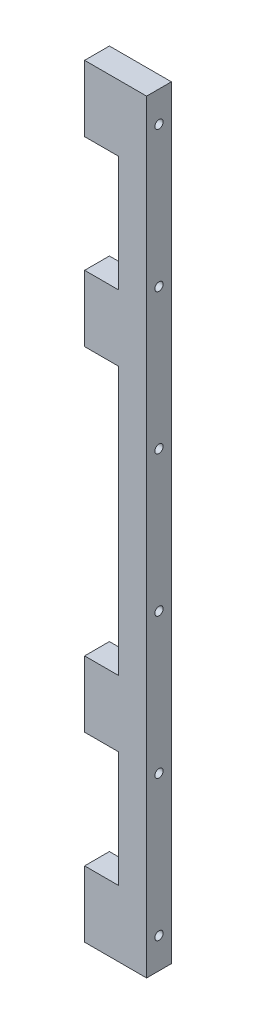
SolidWorks part; units mm, degrees
material "6061-T6"
ref_plane "前视基准面" through (0, 0, 0) normal (0, 0, 1) x (1, 0, 0)
ref_plane "上视基准面" through (0, 0, 0) normal (0, 1, 0) x (1, 0, 0)
ref_plane "右视基准面" through (0, 0, 0) normal (1, 0, 0) x (0, 0, -1)
sketch "草图1" plane through (0, 0, 0) normal (0, 0, 1) x (1, 0, 0)
  line L0 (23.5, 40) -> (23.5, 422) construction
  line L1 (0, 462) -> (40.5, 462)
  line L2 (0, 462) -> (0, 0)
  line L3 (0, 0) -> (40.5, 0)
  line L4 (40.5, 462) -> (40.5, 0)
  line L5 (0, 462) -> (23.5, 462)
  line L6 (0, 462) -> (0, 422)
  line L7 (0, 422) -> (23.5, 422)
  line L8 (23.5, 462) -> (23.5, 422) construction
  line L9 (0, 0) -> (23.5, 0)
  line L10 (0, 0) -> (0, 40)
  line L11 (0, 40) -> (23.5, 40)
  line L12 (23.5, 0) -> (23.5, 40) construction
  line L13 (11.75, 422) -> (11.75, 40) construction
  line L14 (11.75, 231) -> (40.5, 231) construction
  line L15 (23.5, 40) -> (23.5, 422)
  line L16 (0, 352) -> (23.5, 352)
  line L17 (0, 312) -> (23.5, 312)
  line L18 (0, 150) -> (23.5, 150)
  line L19 (0, 110) -> (23.5, 110)
  dimension "D1" = 40.5
  dimension "D2" = 462
  dimension "D3" = 17
  dimension "D4" = 40
  dimension "D5" = 40
  dimension "D6" = 110
  dimension "D7" = 40
  dimension "D8" = 110
extrude "凸台-拉伸1" add sketch "草图1" along normal blind 15 contours L12 L3 L4 L1 L8 L7 L2 L11 | L2 L17 L15 L16 | L2 L19 L15 L18
chamfer "倒角1" distance 3 angle 45 12 edges at (0, 20, 15) (0, 110, 7.5) (0, 150, 7.5) (0, 312, 7.5) (0, 352, 7.5) (0, 422, 7.5) (0, 462, 7.5) (0, 0, 7.5) (0, 40, 7.5) (0, 442, 15) (0, 332, 15) (0, 130, 15)
hole_wizard "M6 螺纹孔1" positions "草图2" profile "草图3" tap size "M6" standard "ISO"
sketch "草图2" plane through (40.5, 0, 0) normal (1, 0, 0) x (0, 0, -1)
  line L0 (-7.5, 18.5) -> (-7.5, 443.5) construction
  line L1 (-7.5, 443.5) -> (-7.5, 462) construction
  line L2 (-15, 462) -> (0, 462) construction
  line L4 (-7.5, 231) -> (0, 231) construction
  line L5 (0, 462) -> (0, 0) construction
  point P0 (-7.5, 443.5)
  point P9 (-7.5, 358.5)
  point P10 (-7.5, 273.5)
  point P11 (-7.5, 188.5)
  point P12 (-7.5, 103.5)
  point P13 (-7.5, 18.5)
  dimension "D2" = 85
  dimension "D1" = 6
cosmetic thread "孔螺蚊线1" parameters "D1"=12, "D2"=6
cosmetic thread "孔螺蚊线2" parameters "D1"=12, "D2"=6
cosmetic thread "孔螺蚊线3" parameters "D1"=12, "D2"=6
cosmetic thread "孔螺蚊线4" parameters "D1"=12, "D2"=6
cosmetic thread "孔螺蚊线5" parameters "D1"=12, "D2"=6
cosmetic thread "孔螺蚊线6" parameters "D1"=12, "D2"=6
sketch "草图3" plane through (40.5, 443.5, 7.5) normal (0, 1, 0) x (0, 0, -1)
  line L0 (0, 0) -> (0, 18.5022)
  line L1 (0, 18.5022) -> (2.5, 17)
  line L2 (2.5, 17) -> (2.5, 0)
  line L5 (2.5, 0) -> (0, 0)
  line L10 (0, 18.5022) -> (-2.5, 17) construction
  line L11 (0, -6.35) -> (0, 107.95) construction
  dimension "螺纹孔钻头直径" = 5
  dimension "螺纹孔钻头深度" = 17
  dimension "导头角度" = 118
